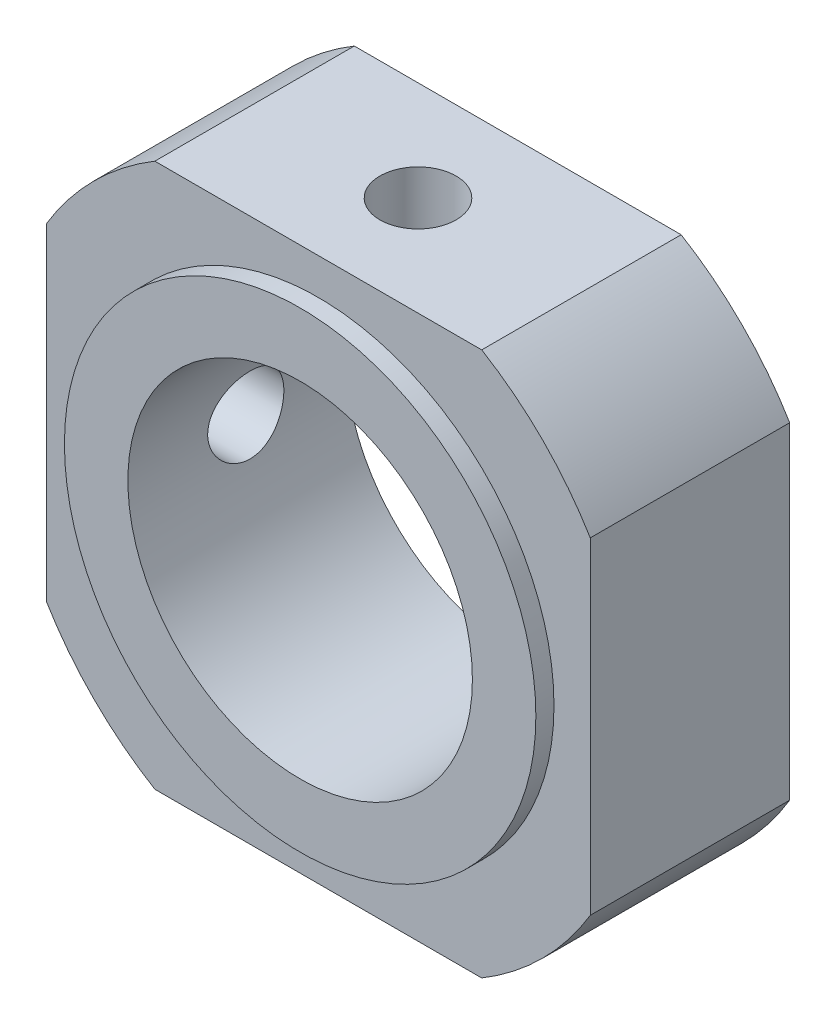
from build123d import *

# Parameters (mm, degrees)
BOSS_EXTRUDE1_DEPTH    = 11
SKETCH2_R              = 13
BOSS_EXTRUDE2_DEPTH    = 1
SKETCH3_R              = 9.5
CUT_EXTRUDE1_DEPTH     = 25.372115214
M5_TAPPED_HOLE1_REACH  = 37.623
M5_TAPPED_HOLE1_BORE_R = 2.1
M5_TAPPED_HOLE2_REACH  = 37.623
M5_TAPPED_HOLE2_BORE_R = 2.1


with BuildPart() as part:
    # Sketch1 → Boss-Extrude1 (new body)
    with BuildSketch(Plane.XY):
        with BuildLine():
            Line((-9.013878189, 15), (9.013878189, 15))
            ThreePointArc((9.013878189, 15), (12.374368671, 12.374368671), (15, 9.013878189))
            Line((15, 9.013878189), (15, -9.013878189))
            ThreePointArc((15, -9.013878189), (12.374368671, -12.374368671), (9.013878189, -15))
            Line((9.013878189, -15), (-9.013878189, -15))
            ThreePointArc((-9.013878189, -15), (-12.374368671, -12.374368671), (-15, -9.013878189))
            Line((-15, -9.013878189), (-15, 9.013878189))
            ThreePointArc((-15, 9.013878189), (-12.374368671, 12.374368671), (-9.013878189, 15))
        make_face()
    extrude(amount=BOSS_EXTRUDE1_DEPTH)

    # Sketch2 → Boss-Extrude2 (add)
    with BuildSketch(Plane.XY.offset(11)):
        Circle(SKETCH2_R)
    extrude(amount=BOSS_EXTRUDE2_DEPTH)

    # Sketch3 → Cut-Extrude1 (cut, through all)
    with BuildSketch(Plane.XY.offset(12)):
        Circle(SKETCH3_R)
    extrude(amount=-CUT_EXTRUDE1_DEPTH, mode=Mode.SUBTRACT)

    # M5 Tapped Hole1 bore → M5 Tapped Hole1 (cut, up to next)
    with BuildSketch(Plane.ZY.offset(15), mode=Mode.PRIVATE) as m5_tapped_hole1_sk1:
        with Locations((5.5, 0)):
            Circle(M5_TAPPED_HOLE1_BORE_R)
    m5_tapped_hole1_tool1 = extrude(m5_tapped_hole1_sk1.sketch, amount=-M5_TAPPED_HOLE1_REACH, mode=Mode.PRIVATE) & part.part
    add(m5_tapped_hole1_tool1.solids().sort_by_distance((-15, 0, 5.5))[0], mode=Mode.SUBTRACT)

    # M5 Tapped Hole2 bore → M5 Tapped Hole2 (cut, up to next)
    with BuildSketch(Plane(origin=(0, 15, 0), x_dir=(-1, 0, 0), z_dir=(0, 1, 0)), mode=Mode.PRIVATE) as m5_tapped_hole2_sk1:
        with Locations((0, 5.5)):
            Circle(M5_TAPPED_HOLE2_BORE_R)
    m5_tapped_hole2_tool1 = extrude(m5_tapped_hole2_sk1.sketch, amount=-M5_TAPPED_HOLE2_REACH, mode=Mode.PRIVATE) & part.part
    add(m5_tapped_hole2_tool1.solids().sort_by_distance((0, 15, 5.5))[0], mode=Mode.SUBTRACT)


solid = part.part
